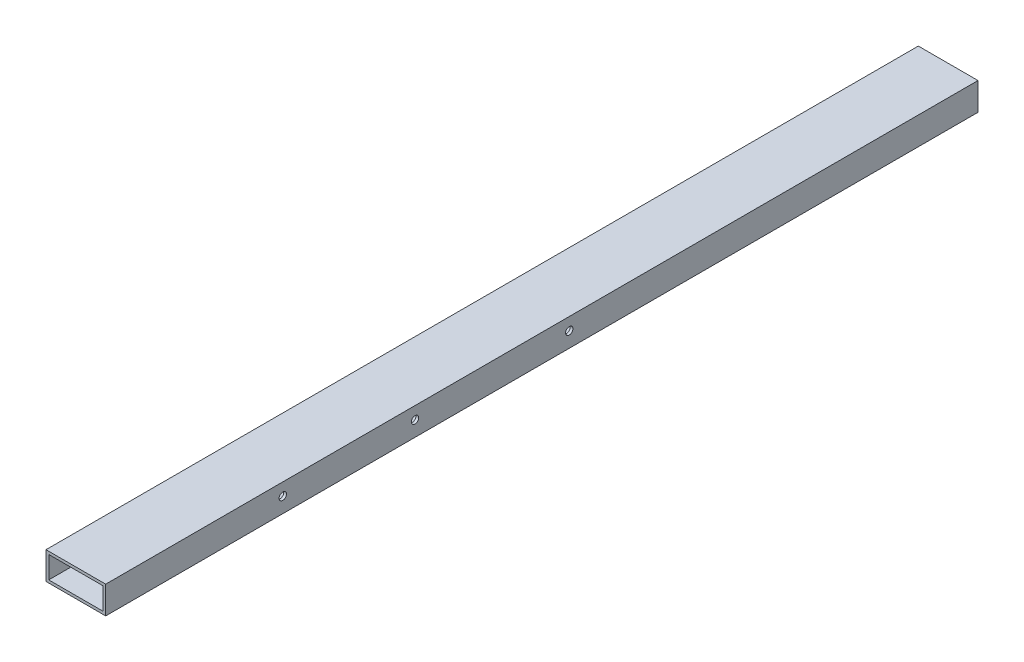
SolidWorks part; units mm, degrees
material "不锈钢管"
ref_plane "Front Plane" through (0, 0, 0) normal (0, 0, 1) x (1, 0, 0)
ref_plane "Top Plane" through (0, 0, 0) normal (0, 1, 0) x (1, 0, 0)
ref_plane "Right Plane" through (0, 0, 0) normal (1, 0, 0) x (0, 0, -1)
other "Configuration Table"
sketch "Sketch1" plane through (0, 0, 0) normal (0, 0, 1) x (1, 0, 0)
  line L0 (-40.5408, 39.808) -> (24.4592, 39.808)
  line L1 (24.4592, 39.808) -> (24.4592, 9.808)
  line L2 (24.4592, 9.808) -> (-40.5408, 9.808)
  line L3 (-40.5408, 9.808) -> (-40.5408, 39.808)
extrude "Boss-Extrude1" add sketch "Sketch1" along normal blind 950
sketch "Sketch2" plane through (0, 0, 950) normal (0, 0, 1) x (1, 0, 0)
  line L0 (-37.5408, 36.808) -> (21.4592, 36.808)
  line L1 (21.4592, 36.808) -> (21.4592, 12.808)
  line L2 (21.4592, 12.808) -> (-37.5408, 12.808)
  line L3 (-37.5408, 12.808) -> (-37.5408, 36.808)
  line L4 (24.4592, 39.808) -> (-40.5408, 39.808) construction
  line L5 (24.4592, 9.808) -> (24.4592, 39.808) construction
  line L6 (-40.5408, 9.808) -> (24.4592, 9.808) construction
  line L7 (-40.5408, 39.808) -> (-40.5408, 9.808) construction
  dimension "D1" = 3
  dimension "D2" = 3
  dimension "D3" = 3
  dimension "D4" = 3
extrude "Cut-Extrude1" cut sketch "Sketch2" against normal blind 950
sketch "Sketch3" plane through (0, 39.808, 0) normal (0, 1, 0) x (1, 0, 0)
  line L0 (-8.0408, 0) -> (-8.0408, -39.0581) construction
  line L1 (24.4592, 0) -> (-40.5408, 0) construction
  circle A0 centre (-8.0408, -39.0581) radius 9.584
sketch "Sketch4" plane through (-40.5408, 0, 0) normal (-1, 0, 0) x (0, 0, 1)
  circle A0 centre (346.1016, 26.308) radius 3
  circle A1 centre (658.1016, 26.308) radius 3
  circle A2 centre (490.1016, 26.308) radius 3
sketch "Sketch5" plane through (-40.5408, 0, 0) normal (-1, 0, 0) x (0, 0, 1)
  circle A0 centre (445.1016, 26.308) radius 4
  circle A1 centre (613.1016, 26.308) radius 4
  circle A2 centre (757.1016, 26.308) radius 4
extrude "Cut-Extrude2" cut sketch "Sketch5" against normal through all
